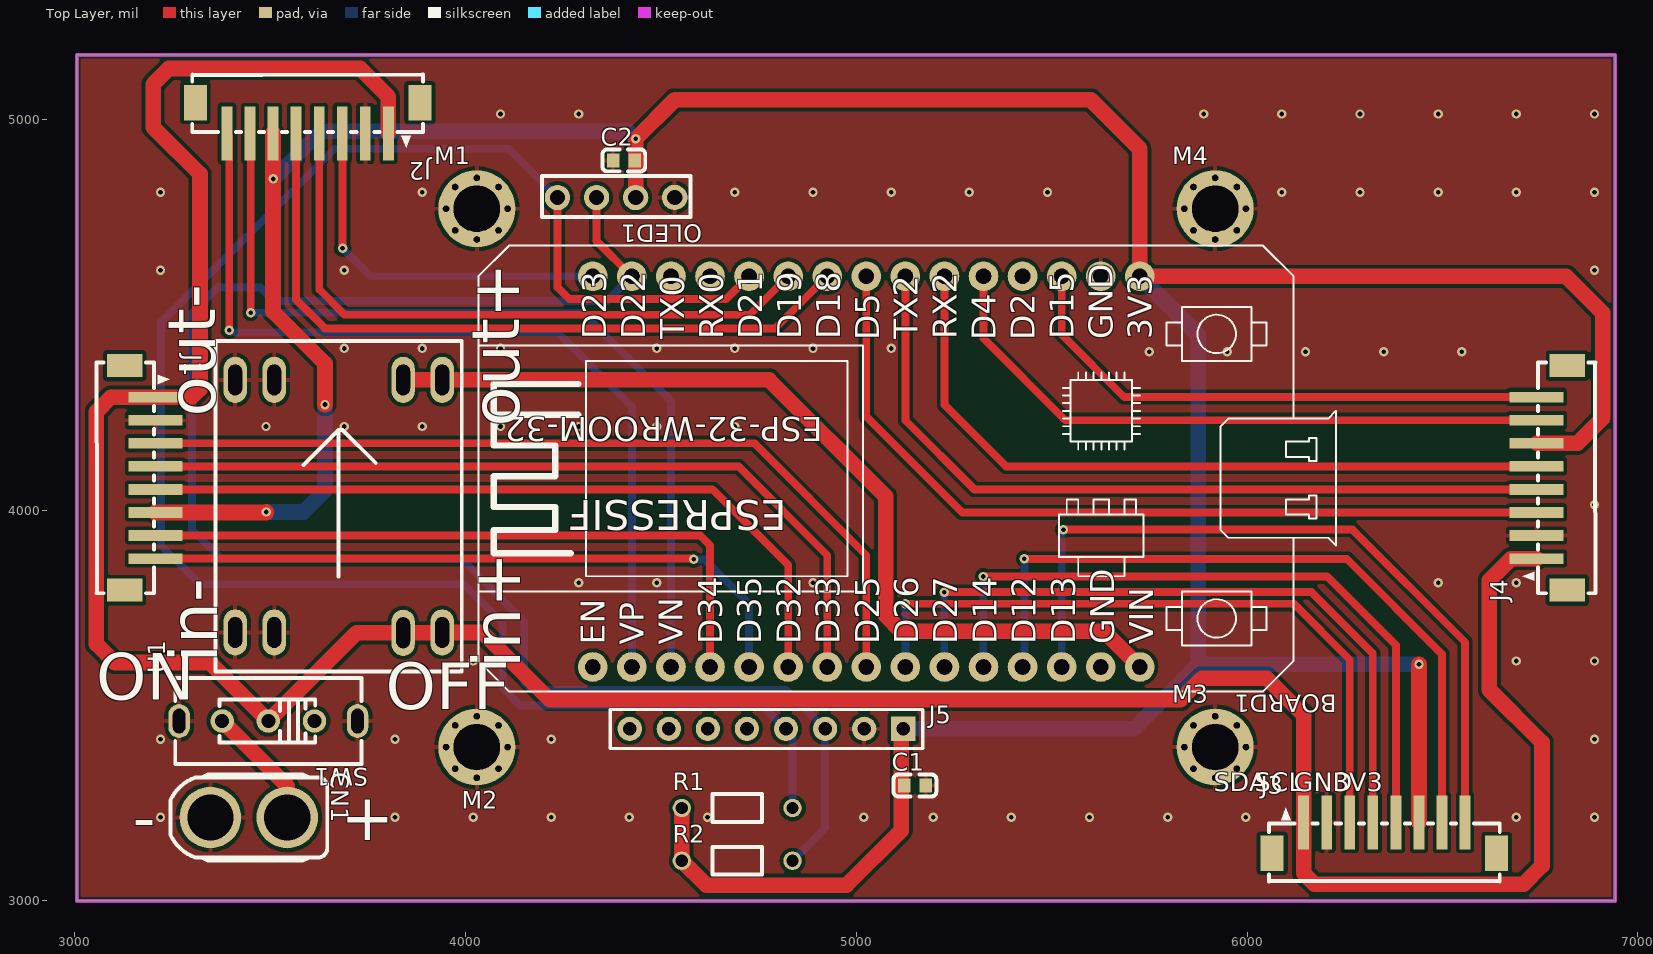
[diagram p0: Top Layer view]
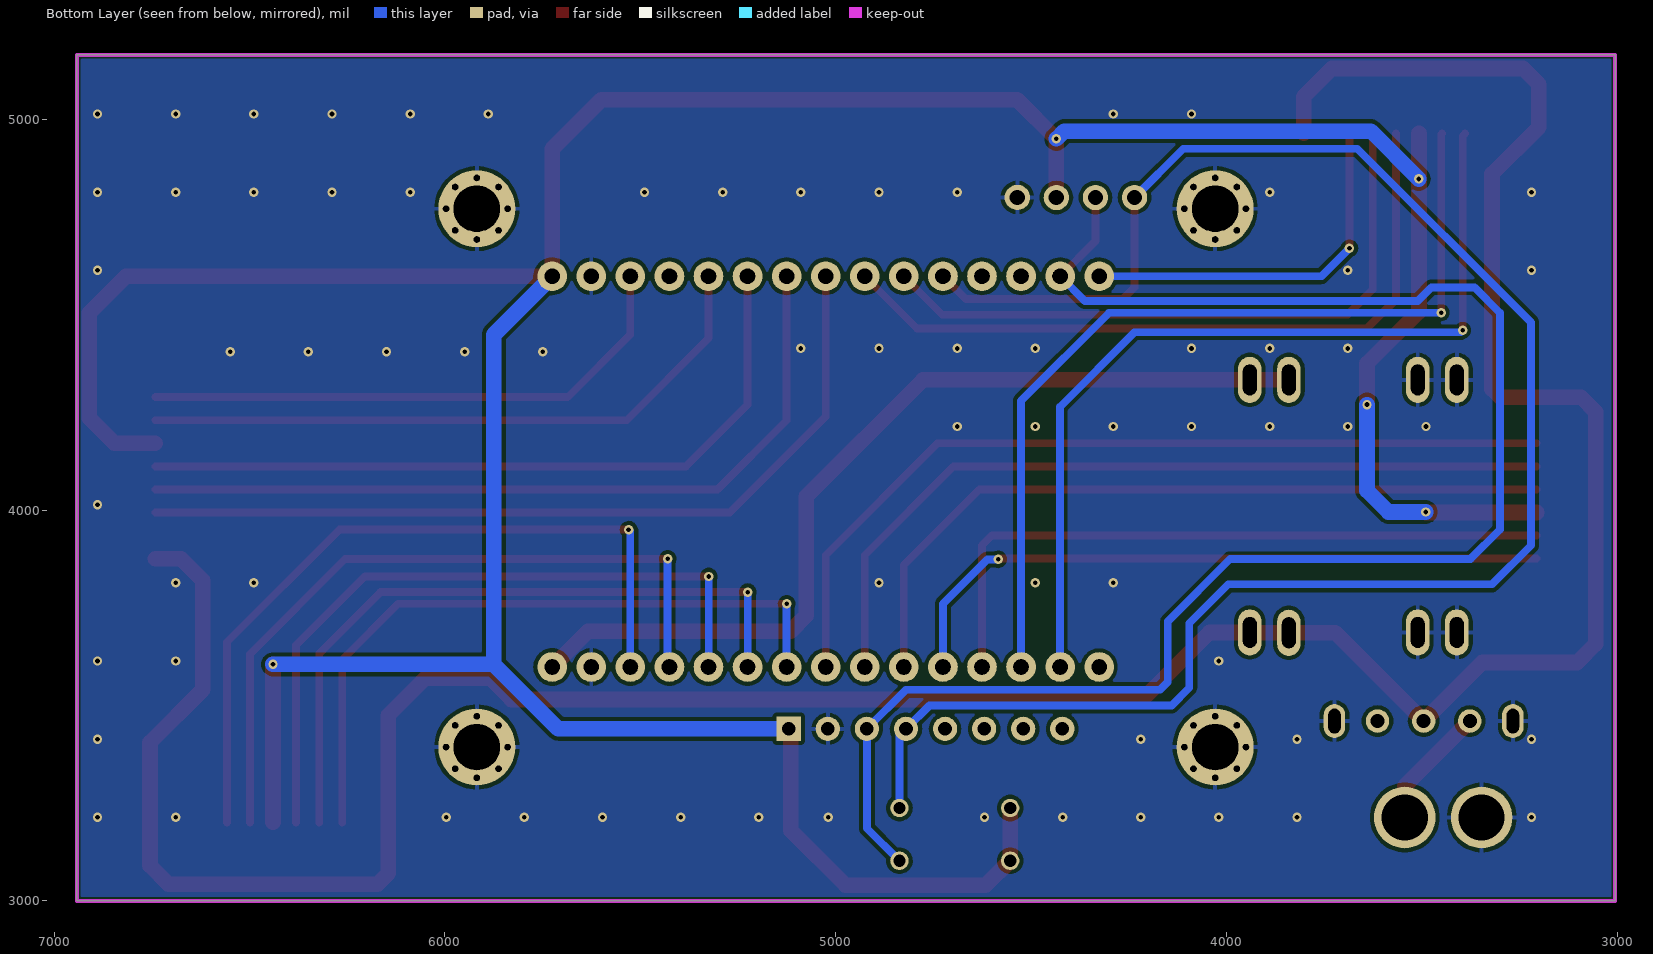
[diagram p1: Bottom Layer view, seen from below]
# Altium PCB MISC89094.pcbdoc
Units mil, origin at the board's own origin, x right, y up, seen from the top; angles counter-clockwise.
Board outline 3937.01 x 2165.35 mil, 2 copper layers (Top Layer, Bottom Layer), stack 62.206 mil thick; 18 components, 27 nets, 141 pads, 83 vias.

## Layer stack, top to bottom
Top Solder Mask Layer: solder mask 0.394, Dk 3.3
Top Layer: signal copper 1.379
Dielectric1: surface 59.449, FR4, Dk 4.5
Bottom Layer: signal copper 1.378
Bottom Solder Mask Layer: solder mask 0.394, Dk 3.3

## Board outline
3005,5165.35 3005,3000 6942.01,3000 6942.01,5165.35

## Design rules (kind name [scope] priority, off if disabled: settings)
BoardOutlineClearance copperThickness2oz_1 [All] p2 off: genericclearance=8 ignorepadtopadclearanceinfootprint=FALSE except(0: Arc-SplitContinuation Track-SplitContinuation SMDPad-SplitContinuation THPad-SplitContinuation Via-SplitContinuation Fill-SplitContinuation Region-SplitContinuation Poly-SplitContinuation Text-SplitContinuation Hole-SplitContinuation; 6: SMDPad-CutoutEdge THPad-CutoutEdge Via-CutoutEdge Fill-CutoutEdge Region-CutoutEdge Text-CutoutEdge Hole-CutoutEdge; 10: Poly-OutlineEdge Poly-CutoutEdge; 11.8: Arc-OutlineEdge Track-OutlineEdge SMDPad-OutlineEdge THPad-OutlineEdge Via-OutlineEdge Fill-OutlineEdge Region-OutlineEdge Text-OutlineEdge Hole-OutlineEdge Arc-CutoutEdge Track-CutoutEdge)
BoardOutlineClearance Plane_innerPlane_1 [All] p4 off: genericclearance=10 ignorepadtopadclearanceinfootprint=FALSE except(0: Arc-SplitContinuation Track-SplitContinuation SMDPad-SplitContinuation THPad-SplitContinuation Via-SplitContinuation Fill-SplitContinuation Region-SplitContinuation Poly-SplitContinuation Text-SplitContinuation Hole-SplitContinuation; 5.98: SMDPad-CutoutEdge THPad-CutoutEdge Via-CutoutEdge Fill-CutoutEdge Region-CutoutEdge Text-CutoutEdge Hole-CutoutEdge; 10: Poly-OutlineEdge Poly-CutoutEdge; 11.81: Arc-OutlineEdge Track-OutlineEdge SMDPad-OutlineEdge THPad-OutlineEdge Via-OutlineEdge Fill-OutlineEdge Region-OutlineEdge Text-OutlineEdge Hole-OutlineEdge Arc-CutoutEdge Track-CutoutEdge)
BoardOutlineClearance Copper_copperRegion_1 [All] p6 off: genericclearance=10 ignorepadtopadclearanceinfootprint=FALSE except(0: Arc-SplitContinuation Track-SplitContinuation SMDPad-SplitContinuation THPad-SplitContinuation Via-SplitContinuation Fill-SplitContinuation Region-SplitContinuation Poly-SplitContinuation Text-SplitContinuation Hole-SplitContinuation; 5.98: SMDPad-CutoutEdge THPad-CutoutEdge Via-CutoutEdge Fill-CutoutEdge Region-CutoutEdge Text-CutoutEdge Hole-CutoutEdge; 10: Poly-OutlineEdge Poly-CutoutEdge; 11.81: Arc-OutlineEdge Track-OutlineEdge SMDPad-OutlineEdge THPad-OutlineEdge Via-OutlineEdge Fill-OutlineEdge Region-OutlineEdge Text-OutlineEdge Hole-OutlineEdge Arc-CutoutEdge Track-CutoutEdge)
BoardOutlineClearance copperThickness1oz_1 [All] p8: genericclearance=10 ignorepadtopadclearanceinfootprint=FALSE except(0: Arc-SplitContinuation Track-SplitContinuation SMDPad-SplitContinuation THPad-SplitContinuation Via-SplitContinuation Fill-SplitContinuation Region-SplitContinuation Poly-SplitContinuation Text-SplitContinuation Hole-SplitContinuation; 5.98: SMDPad-CutoutEdge THPad-CutoutEdge Via-CutoutEdge Fill-CutoutEdge Region-CutoutEdge Text-CutoutEdge Hole-CutoutEdge; 10: Poly-OutlineEdge Poly-CutoutEdge; 11.81: Arc-OutlineEdge Track-OutlineEdge SMDPad-OutlineEdge THPad-OutlineEdge Via-OutlineEdge Fill-OutlineEdge Region-OutlineEdge Text-OutlineEdge Hole-OutlineEdge Arc-CutoutEdge Track-CutoutEdge)
Clearance copperThickness2oz [All] p1 off: gap=8 ignorepadtopadclearanceinfootprint=FALSE except(6: SMDPad-Track SMDPad-SMDPad THPad-Track SMDPad-THPad THPad-THPad Track-Via SMDPad-Via THPad-Via Via-Via Fill-Track Region-Track Fill-SMDPad Region-SMDPad Fill-THPad Region-THPad Fill-Via Region-Via Fill-Fill Fill-Region Region-Region Arc-Track Arc-SMDPad Arc-THPad Arc-Via Fill-Arc Region-Arc Arc-Arc Text-Track SMDPad-Text Text-THPad Text-Via Fill-Text Region-Text Arc-Text Text-Text Hole-Track Hole-SMDPad Hole-THPad Hole-Via Fill-Hole Region-Hole Hole-Arc Hole-Text; 10: Poly-Track Poly-SMDPad Poly-THPad Poly-Via Poly-Fill Poly-Region Poly-Poly Poly-Arc Poly-Text Poly-Hole)
Clearance Plane_innerPlane [All] p3 off: gap=10 ignorepadtopadclearanceinfootprint=FALSE except(5.98: SMDPad-SMDPad SMDPad-THPad THPad-THPad Track-Via SMDPad-Via THPad-Via Via-Via Fill-Track Region-Track Fill-SMDPad Region-SMDPad Fill-THPad Region-THPad Fill-Via Region-Via Fill-Fill Fill-Region Region-Region Arc-Track Arc-SMDPad Arc-THPad Arc-Via Fill-Arc Region-Arc Arc-Arc Text-Track SMDPad-Text Text-THPad Text-Via Fill-Text Region-Text Arc-Text Text-Text Hole-SMDPad Hole-THPad Hole-Via Fill-Hole Region-Hole Hole-Arc Hole-Text; 6: SMDPad-Track THPad-Track Hole-Track)
Clearance Copper_copperRegion [All] p5 off: gap=10 ignorepadtopadclearanceinfootprint=FALSE except(5.98: SMDPad-SMDPad SMDPad-THPad THPad-THPad Track-Via SMDPad-Via THPad-Via Via-Via Fill-Track Region-Track Fill-SMDPad Region-SMDPad Fill-THPad Region-THPad Fill-Via Region-Via Fill-Fill Fill-Region Region-Region Arc-Track Arc-SMDPad Arc-THPad Arc-Via Fill-Arc Region-Arc Arc-Arc Text-Track SMDPad-Text Text-THPad Text-Via Fill-Text Region-Text Arc-Text Text-Text Hole-SMDPad Hole-THPad Hole-Via Fill-Hole Region-Hole Hole-Arc Hole-Text; 6: SMDPad-Track THPad-Track Hole-Track)
Clearance copperThickness1oz [All] p7: gap=10 ignorepadtopadclearanceinfootprint=FALSE except(5.98: SMDPad-SMDPad SMDPad-THPad THPad-THPad Track-Via SMDPad-Via THPad-Via Via-Via Fill-Track Region-Track Fill-SMDPad Region-SMDPad Fill-THPad Region-THPad Fill-Via Region-Via Fill-Fill Fill-Region Region-Region Arc-Track Arc-SMDPad Arc-THPad Arc-Via Fill-Arc Region-Arc Arc-Arc Text-Track SMDPad-Text Text-THPad Text-Via Fill-Text Region-Text Arc-Text Text-Text Hole-SMDPad Hole-THPad Hole-Via Fill-Hole Region-Hole Hole-Arc Hole-Text; 6: SMDPad-Track THPad-Track Hole-Track)
DiffPairsRouting differentialPair [All] p1: maxlimit=6 minlimit=6 mostfreqgap=6 toplayer_minwidth=5 toplayer_prefwidth=10 toplayer_maxwidth=100 toplayer_mingap=6 toplayer_prefgap=6 toplayer_maxgap=6 bottomlayer_minwidth=5 bottomlayer_prefwidth=10 bottomlayer_maxwidth=100 bottomlayer_mingap=6 bottomlayer_prefgap=6 bottomlayer_maxgap=6 maxuncoupledlength=10
HoleToHoleClearance otherClearance [All] p1: gap=11.8 allowstackedmicrovias=TRUE
Length netLength [All] p1: minlimit=0 maxlimit=0
PasteMaskExpansion pasteMaskExpansion [All] p1: expansion=0
PlaneConnect innerPlane [All] p1: planeconnectstyle=Relief reliefexpansion=20 reliefentries=4 reliefconductorwidth=10 reliefairgap=10
PolygonConnect copperRegion [All] p1: connectstyle=Relief reliefconductorwidth=10 reliefentries=4 polygonreliefangle="90 Angle" airgapwidth=10 via.connectstyle=Relief via.reliefconductorwidth=10 via.reliefentries=4 via.polygonreliefangle="90 Angle" via.airgapwidth=10
RoutingVias viaSize [All] p1: holewidth=12 width=24 viastyle="Through Hole" minholewidth=11.8 minwidth=19.7 maxholewidth=248 maxwidth=393.7
SolderMaskExpansion solderMaskExpansion [IsVia] p1: expansion=-1000 istentingtop=TRUE
SolderMaskExpansion solderMaskExpansion [All] p2: expansion=2 istentingtop=FALSE
Width copperThickness2oz_2 [All] p1 off: maxlimit=100 minlimit=8 preferedwidth=10
Width copperThickness1oz_2 [All] p2: maxlimit=100 minlimit=5 preferedwidth=10

## Components (designator, comment, footprint, x,y, rotation, side; value= is the part's Value field where it differs from the comment)
BOARD1 "ESP32DEVKITV1 COPY" ESP32-DEVKITV1 5130,4155.35 r180 top
C1 "100nF" C0603 5150,3295.35 r0 top
C2 "100nF" C0603 4405,4895.35 r0 top
CN1 "XT30UPB-F" XT30 3445,3213.5 r270 top
J1 "zh1.5-8p" ZH1.5-8P 3162.48,4082.68 r270 top
J2 "zh1.5-8p" ZH1.5-8P 3595.55,5007.87 r180 top
J3 "zh1.5-8p" ZH1.5-8P 6351.46,3157.48 r0 top
J4 "zh1.5-8p" ZH1.5-8P 6784.53,4082.68 r90 top
J5 "HDR-M-2.54_1x8" HDR-M-2.54_1X8 4720,3440.35 r180 top
M1 "M3" M3 4028.62,4771.38 r0 top
M2 "M3" M3 4028.62,3393.42 r0 top
M3 "M3" M3 5918.39,3393.42 r0 top
M4 "M3" M3 5918.39,4771.38 r0 top
OLED1 "0.96OLED_4P_MODULE_JX" 0.96OLED_4P 4385,4800.35 r180 top
R1 "4.7kΩ" Res_1/8W 4695,3235.35 r0 top
R2 "4.7kΩ" Res_1/8W 4695,3100.35 r0 top
SW1 "SS-12F44-G6" SW-TH_SS-12F44-GX 3495,3460.35 r180 top
U1 "5v_buck" 5V_BUCK 3675,4010.35 r90 top

## Footprints (in the part's own frame and the unit in brackets; to place one, negate y for a bottom-side part, rotate by r counter-clockwise, add the part's x,y. Pads: shape width x height; smd on the part's side, far side on the other; paste and mask are expansions set on the pad)
0.96OLED_4P [mm]
  round 1.65 hole 1 paste+0 mask+0.051: 1(-3.81,-0.001) 2(-1.27,0.002) 3(1.27,0.002) 4(3.81,0.002)
  silkscreen extent -4.83,-1.4 4.83,1.27
5V_BUCK [mm]
  oval 3x1.524 hole 0.9 slot 2 at 0 deg paste+0 mask+0.051: 1(-8.21,4.19) 1(-8.21,6.73) 2(-8.232,-4.19) 2(-8.21,-6.73) 3(8.21,6.73) 3(8.21,4.19) 4(8.21,-6.73) 4(8.21,-4.19)
  silkscreen extent -10.75,-8 10.75,8
C0603 [mm]
  rect 0.8x0.9 smd: 1(-0.7,0) 2(0.7,0)
  silkscreen extent -1.39,-0.71 1.39,0.71
ESP32-DEVKITV1 [mil]
  round 76 hole 39.36 paste+4 mask+4: 3V3(-595.47,-443.38) D2(-295.47,-443.38) D4(-195.47,-443.38) D5(104.53,-443.38) D12(-295.47,556.62) D13(-395.47,556.62) D14(-195.47,556.62) D15(-395.47,-443.38) D18(204.53,-443.38) D19(304.53,-443.37) D21(404.53,-443.37) D22(704.53,-443.37) D23(804.53,-443.37) D25(104.53,556.62) D26(4.53,556.62) D27(-95.47,556.62) D32(304.53,556.62) D33(204.53,556.62) D34(504.53,556.63) D35(404.53,556.62) EN(804.53,556.63) GND(-495.47,556.62) GND1(-495.47,-443.38) VIN(-595.47,556.62) VN(604.53,556.63) VP(704.53,556.63)
  round 76 hole 39.36 paste+0 mask+4: RX0(504.53,-443.37) RX2(-95.47,-443.38) TX0(604.53,-443.37) TX2(4.53,-443.38)
  silkscreen extent -1097,-522 1097,620
HDR-M-2.54_1X8 [mil]
  rect 62x62 hole 35 paste+0 mask+2: 1(-400,0)
  round 62 hole 35 paste+0 mask+2: 2(-300,0) 3(-200,0) 4(-100,0) 5(0,0) 6(100,0) 7(200,0) 8(300,0)
  silkscreen extent -450,-50 350,50
M3 [mm]
  round 0.6 hole 0.4 slot 0.405 at 0 deg paste+0 mask+0.051: 1(-2,0.007) 1(-1.41,-1.403) 1(-1.41,1.417) 1(0,-1.993) 1(0,2.007) 1(1.41,-1.403) 1(1.41,1.417) 1(2,0.007)
  round 5 hole 3 slot 3.005 at 0 deg paste+0 mask+0.051: 1(0,0.007)
Res_1/8W [mil]
  round 47.2 hole 31.5 paste+0 mask+2: 1(-141.7,2.48) 2(141.7,2.48)
  silkscreen extent -63,-33 63,38
SW-TH_SS-12F44-GX [mm]
  round 1.524 hole 0.914 paste+0 mask+0.051: 1(-3,0) 2(0,0) 3(3,0)
  oval 1.4x2.2 hole 0.8 slot 1.6 at 90 deg paste+0 mask+0.051: 4(5.8,0) 5(-5.8,0)
  silkscreen extent -6.05,-2.8 6.05,2.8
XT30 [mm]
  round 4 hole 3 paste+0 mask+0.102: 1(0,2.5) 2(0,-2.5)
  silkscreen extent -2.8,-5.1 2.8,5.1
ZH1.5-8P [mm]
  rect 0.7x3.5 smd paste+0 mask+0.051: 1(-5.25,1.104) 2(-3.75,1.104) 3(-2.25,1.104) 4(-0.75,1.104) 5(0.75,1.104) 6(2.25,1.104) 7(3.75,1.104) 8(5.25,1.104)
  rect 1.5x2.3 smd paste+0 mask+0.051: 9(7.3,-0.896) 10(-7.3,-0.896)
  silkscreen extent -7.5,-2.73 7.5,2.04

## Via types
v1: diameter 24, hole 12, Top Layer to Bottom Layer, 69 vias
v2: diameter 24.02, hole 12, Top Layer to Bottom Layer, 14 vias

## Nets (pads, with @x,y where several pads share a name; then routed paths per layer and width w, separated by ;. In a path a pad name is that pad's centre, name@x,y a point inside that pad or via, vN(x,y) a via of type N, cw(c..) or ccw(c..) an arc to the next point about the centre after c; other vN are vias at no path point)
3V3: BOARD1.3V3 C1.1 C2.2 J1.6 J2.6 J3.6 J4.6 J5.1 OLED1.2 R1.1 R2.1 | length 9853.3
  Top Layer w40: J1.6 3490,3994.1 v2(3490,3995.35) ; J2.6 3506.97,4508.38 3640,4375.35 v2(3640,4270.35) ; OLED1.2 v2(4435.01,4950.36) 4535,5050.35 5600,5050.35 5725.47,4924.88 BOARD1.3V3 6816.62,4598.73 6910,4505.35 6910,4235.35 6845.9,4171.26 J4.6 ; R1.1 R2.1 4615.78,3040.35 4975,3040.35 5115,3180.35 5115,3435.35 J5.1 ; J3.6 v2(6440.04,3605.35)
  Bottom Layer w40: v2(3490,3995.35) 3585,3995.35 3640,4050.35 v2(3640,4270.35) ; v2(3507.5,4847.85) 3630,4970.35 4415.01,4970.35 v2(4435.01,4950.36) ; J5.1 5710,3440.35 5875,3605.35 ; BOARD1.3V3 5875,4449.2 5875,3605.35 ; v2(6440.04,3605.35) 5875,3605.35
$1N918: CN1.1 SW1.3 | length 315.8
  Top Layer w40: SW1.3 3543.41,3293.84 CN1.1
+5V: BOARD1.VIN U1.4 | length 2368.6
  Top Layer w40: U1.4@3839.97,4333.58 3939.96,4333.58 4776.77,4333.58 5075,4035.35 5075,3730.35 5115,3690.35 5633.85,3690.35 BOARD1.VIN
GND: BOARD1.GND BOARD1.GND1 C1.2 C2.1 CN1.2 J1.2 J2.2 J3.2 J4.2 J5.2 M1.1 M2.1 M3.1 M4.1 OLED1.1 SW1.4 SW1.5 U1.1 U1.3
  other v1: 3219.1,3214.1 3819.1,3214.1 4019.1,3214.1 4219.1,3214.1 4419.1,3214.1 4619.1,3214.1 5019.1,3214.1 5196.76,3214.1 5396.76,3214.1 5596.76,3214.1 5796.76,3214.1 5996.76,3214.1 6689.1,3214.1 6889.1,3214.1 3219.1,3414.1 3819.1,3414.1 4219.1,3414.1 6889.1,3414.1 4019.1,3614.1 6689.1,3614.1 6889.1,3614.1 4289.1,3814.1 4489.1,3814.1 4889.1,3814.1 6489.1,3814.1 6689.1,3814.1 6889.1,4014.1 3489.1,4214.1 3689.1,4214.1 3889.1,4214.1 4089.1,4214.1 4289.1,4214.1 4489.1,4214.1 4689.1,4214.1 5749.57,4405.36 5949.57,4405.36 6149.57,4405.36 6349.57,4405.36 6549.57,4405.36 3689.1,4414.1 3889.1,4414.1 4089.1,4414.1 4489.1,4414.1 4689.1,4414.1 4889.1,4414.1 5089.1,4414.1 3219.1,4614.1 3689.1,4614.1 6889.1,4614.1 3219.1,4814.1 3889.1,4814.1 4689.1,4814.1 4889.1,4814.1 5089.1,4814.1 5289.1,4814.1 5489.1,4814.1 6089.1,4814.1 6289.1,4814.1 6489.1,4814.1 6689.1,4814.1 6889.1,4814.1 4089.1,5014.1 4289.1,5014.1 5889.1,5014.1 6089.1,5014.1 6289.1,5014.1 6489.1,5014.1 6689.1,5014.1 6889.1,5014.1
M1BRK: BOARD1.D25 J1.3 | length 2224.3
  Top Layer w20: J1.3 4739.1,4171.26 5025.47,3884.88 BOARD1.D25
M1DIR: BOARD1.D32 J1.5 | length 1960.7
  Top Layer w20: J1.5 4632.2,4053.15 4825.47,3859.88 BOARD1.D32
M1ENCODER1: BOARD1.D34 J1.7 | length 1741.1
  Top Layer w20: J1.7 4600.31,3935.05 4625.47,3909.88 BOARD1.D34
M1ENCODER2: BOARD1.D35 J1.8 | length 1728.8
  Top Layer w20: J1.8 4581.94,3875.99 v2(4583.79,3874.14)
  Bottom Layer w20: v2(4583.79,3874.14) 4611.21,3874.14 4725.47,3759.88 BOARD1.D35
M1PWM: BOARD1.D33 J1.4 | length 2099.8
  Top Layer w20: J1.4 4698.15,4112.21 4925.47,3884.88 BOARD1.D33
M2BRK: BOARD1.D23 J2.3 | length 964.5
  Top Layer w20: J2.3 3685,4963.54 v2(3685,4670.35)
  Bottom Layer w20: v2(3685,4670.35) 3756.62,4598.73 BOARD1.D23
M2DIR: BOARD1.D18 J2.5 | length 1870.4
  Top Layer w20: J2.5 3566.03,4539.33 3640,4465.35 4792.1,4465.35 BOARD1.D18
M2ENCODER1: BOARD1.VN J2.7 | length 2309.9
  Top Layer w20: J2.7 3450,4962.33 v2(3450,4505.35)
  Bottom Layer w20: v2(3450,4505.35) 4300,4505.35 4525.47,4279.88 BOARD1.VN
M2ENCODER2: BOARD1.VP J2.8 | length 2284.2
  Top Layer w20: J2.8 3395,4958.27 v2(3395,4460.35)
  Bottom Layer w20: v2(3395,4460.35) 3400,4455.35 4235,4455.35 4425.47,4264.88 BOARD1.VP
M2PWM: BOARD1.D19 J2.4 | length 1667.2
  Top Layer w20: J2.4 3625.08,4565.27 3690,4500.35 4727.1,4500.35 BOARD1.D19
M3BRK: BOARD1.D26 J3.3 | length 1774.7
  Top Layer w20: v2(5125.47,3760.35) 6120,3760.35 6262.88,3617.48 J3.3
  Bottom Layer w20: BOARD1.D26 v2(5125.47,3760.35)
M3DIR: BOARD1.D14 J3.5 | length 1814.1
  Top Layer w20: v2(5325,3830.35) 6205,3830.35 6380.98,3654.37 J3.5
  Bottom Layer w20: v2(5325,3830.35) 5325,3599.2 BOARD1.D14
M3ENCODER1: BOARD1.D12 J3.7 | length 1879
  Top Layer w20: v2(5430,3875.35) 6255,3875.35 6499.09,3631.27 J3.7
  Bottom Layer w20: BOARD1.D12 5430,3603.26 v2(5430,3875.35)
M3ENCODER2: BOARD1.D13 J3.8 | length 1962.3
  Top Layer w20: v2(5530,3950.35) 6270,3950.35 6558.14,3662.21 J3.8
  Bottom Layer w20: BOARD1.D13 5525.47,3945.82 v2(5530,3950.35)
M3PWM: BOARD1.D27 J3.4 | length 1786.2
  Top Layer w20: v2(5225,3790.35) 6165,3790.35 6321.93,3633.43 J3.4
  Bottom Layer w20: v2(5225,3790.35) 5225,3599.2 BOARD1.D27
M4BRK: BOARD1.D5 J4.3 | length 2176.2
  Top Layer w20: BOARD1.D5 5025.47,4239.88 5271.26,3994.1 J4.3
M4DIR: BOARD1.RX2 J4.5 | length 1909.7
  Top Layer w20: BOARD1.RX2 5225.47,4269.88 5383.15,4112.2 J4.5
M4ENCODER1: BOARD1.D4 J4.7 | length 1661.2
  Top Layer w20: BOARD1.D4 5325.47,4439.88 5535.05,4230.31 J4.7
M4ENCODER2: BOARD1.D15 J4.8 | length 1430.9
  Top Layer w20: BOARD1.D15 5525.47,4449.88 5685.99,4289.36 J4.8
M4PWM: BOARD1.TX2 J4.4 | length 2057.6
  Top Layer w20: BOARD1.TX2 5125.47,4229.88 5302.21,4053.15 J4.4
SCL: BOARD1.D22 J5.3 OLED1.3 R2.2 | length 4281.2
  Top Layer w20: OLED1.3 4335.01,4689.19 BOARD1.D22
  Bottom Layer w20: BOARD1.D22 4362.1,4535.35 3510,4535.35 3475,4570.35 3365,4570.35 3300,4505.35 3300,3950.35 3375,3875.35 3990,3875.35 4150,3715.35 4150,3560.35 4170,3540.35 4820,3540.35 J5.3 4920,3186.13 R2.2
SDA: BOARD1.D21 J5.4 OLED1.4 R1.2 | length 4678.9
  Top Layer w20: OLED1.4 4235,4570.35 4265,4540.35 4667.1,4540.35 BOARD1.D21
  Bottom Layer w20: OLED1.4 4109.94,4925.35 3665,4925.35 3220,4480.35 3220,3910.35 3320,3810.35 3995,3810.35 4095,3710.35 4095,3545.35 4140,3500.35 4760,3500.35 J5.4 4836.7,3423.65 R1.2
VBAT: J1.1 J2.1 J3.1 J4.1 SW1.2 U1.2 | length 7831.1
  Top Layer w40: J2.1 3802.24,5058.11 3730,5130.35 3240,5130.35 3200,5090.35 3200,4980.35 3320,4860.35 3320,4310.35 3299.01,4289.37 J1.1 3092.2,4289.37 3055,4252.17 3055,3657.17 3101.81,3610.35 3345,3610.35 SW1.2 3720.89,3686.24 3839.96,3686.24 3939.08,3686.24 3939.96,3687.12 4043.23,3687.12 4215,3515.35 5830,3515.35 5885,3570.35 6050,3570.35 6144.77,3475.59 J3.1 6144.77,3070.59 6172.5,3042.85 6707.5,3042.85 6755,3090.35 6755,3405.35 6620,3540.35 6620,3820.35 6675.63,3875.99 J4.1
pads on no net: BOARD1.D2 BOARD1.EN BOARD1.RX0 BOARD1.TX0 J1.9 J1.10 J2.9 J2.10 J3.9 J3.10 J4.9 J4.10 J5.5 J5.6 J5.7 J5.8 SW1.1

## Polygon pours and split planes (outlines as drawn)
GND on Bottom Layer (solid, remove dead copper, pour order 2): 3005,5165.35 6940,5165.35 6945,5160.35 6945,3010.35 6940,3005.35 3005,3005.35
GND on Top Layer (solid, remove dead copper, pour order 2): 3005,5165.35 6942.01,5165.35 6942.01,3007.36 6940,3005.35 3005,3005.35 3000,3010.35 3000,5160.35

## Keep-outs
Board Outline Layer:
  the board outline again, w10

## Silkscreen, mask and mechanical layers (free items; w line width, h text height)
Top Silkscreen Layer:
  text "ON" at 3055,3515.35 h120
  text "OFF" at 3795,3490.35 h120
  text "SDA" at 5915,3280.35 h48
  text "SCL" at 6020,3280.35 h48
  text "GND" at 6120,3280.35 h48
  text "3V3" at 6220,3280.35 h48
  text "-" at 3148.27,3155.35 h120
  text "+" at 3680,3155.35 h120